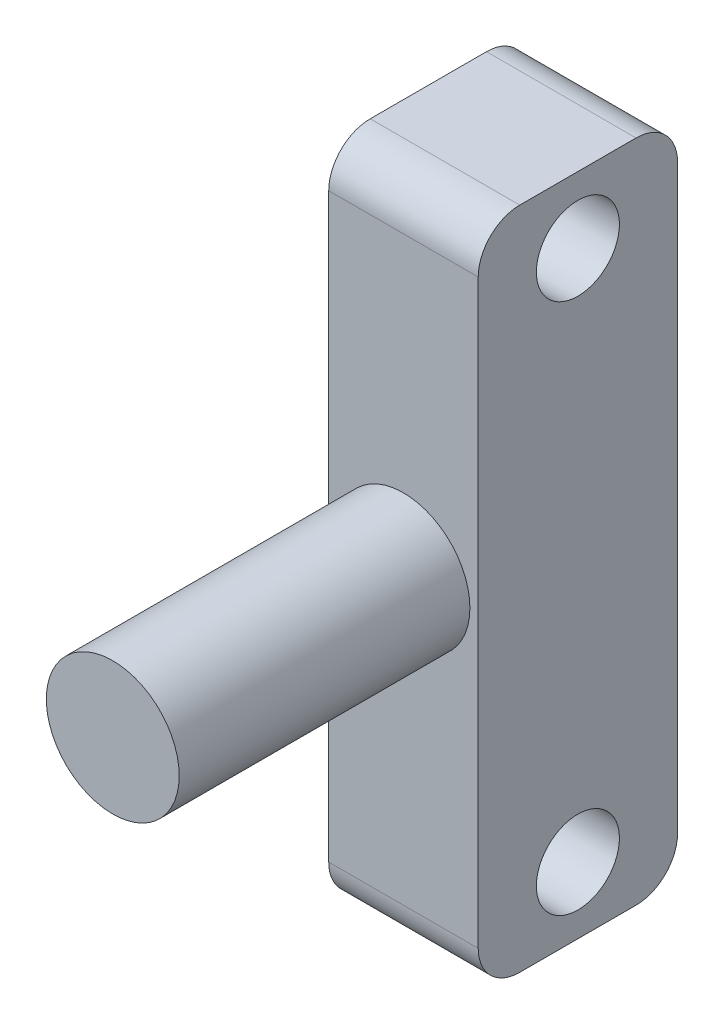
from build123d import *

# Parameters (mm, degrees)
SKETCH1_R           = 8
BOSS_EXTRUDE1_DEPTH = 35
SKETCH2_W           = 18
SKETCH2_H           = 80
BOSS_EXTRUDE2_DEPTH = 24
FILLET1_R           = 5
SKETCH4_R           = 5
CUT_EXTRUDE1_DEPTH  = 57.115951386


with BuildPart() as part:
    # Sketch1 → Boss-Extrude1 (new body)
    with BuildSketch(Plane.XY):
        Circle(SKETCH1_R)
    extrude(amount=BOSS_EXTRUDE1_DEPTH)

    # Sketch2 → Boss-Extrude2 (add)
    with BuildSketch(Plane(origin=(0, 0, 0), x_dir=(-1, 0, 0), z_dir=(0, 0, -1))):
        Rectangle(SKETCH2_W, SKETCH2_H)
    extrude(amount=BOSS_EXTRUDE2_DEPTH)

    # Fillet1
    fillet1_edges = [part.edges().sort_by_distance(p)[0] for p in [
        (0, -40, 0),
        (0, 40, 0),
        (0, -40, -24),
        (0, 40, -24),
    ]]
    fillet(fillet1_edges, radius=FILLET1_R)

    # Sketch4 → Cut-Extrude1 (cut, through all)
    with BuildSketch(Plane.ZY.offset(9)):
        with Locations(Location((-12, -32, 0), (0, 0, 270))):
            Circle(SKETCH4_R)
        with Locations(Location((-12, 32, 0), (0, 0, 270))):
            Circle(SKETCH4_R)
    extrude(amount=-CUT_EXTRUDE1_DEPTH, mode=Mode.SUBTRACT)


solid = part.part
